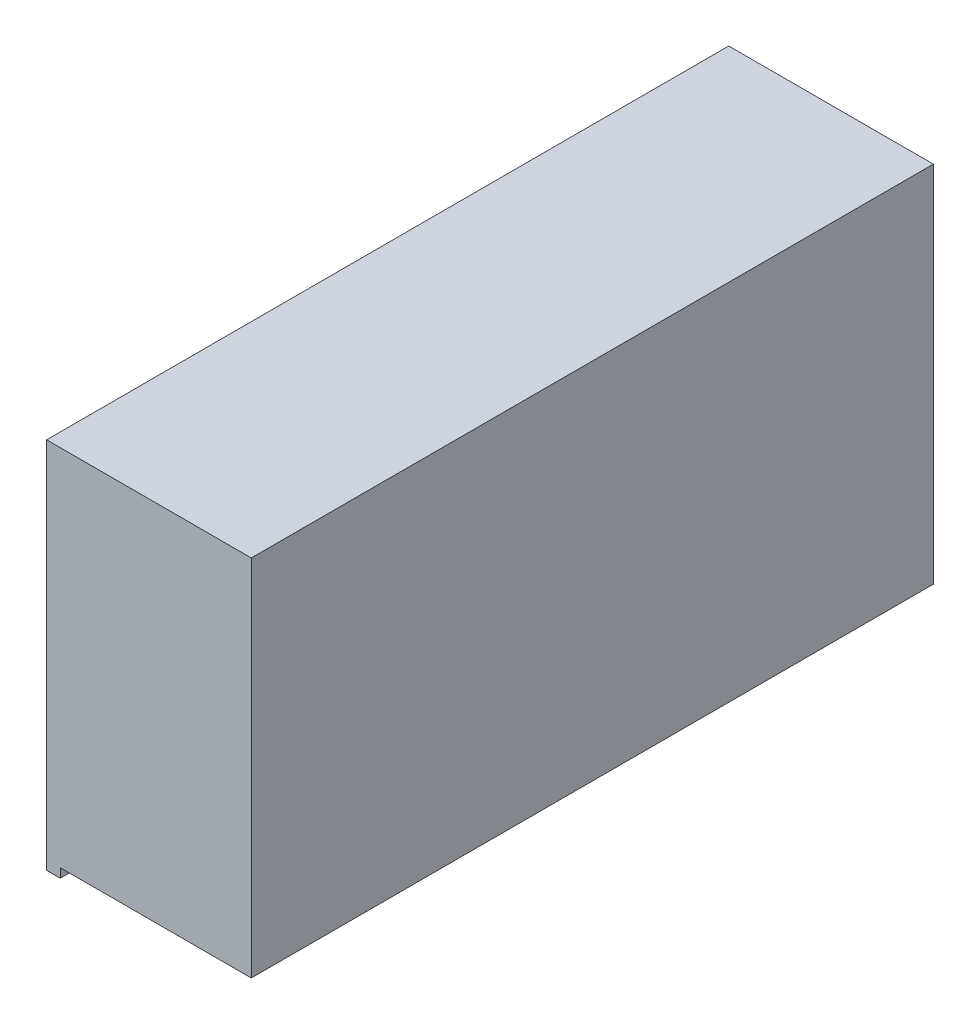
SolidWorks part; units mm, degrees
ref_plane "前视基准面" through (0, 0, 0) normal (0, 0, 1) x (1, 0, 0)
ref_plane "上视基准面" through (0, 0, 0) normal (0, 1, 0) x (1, 0, 0)
ref_plane "右视基准面" through (0, 0, 0) normal (1, 0, 0) x (0, 0, -1)
sketch "草图1" plane through (0, 0, 0) normal (0, 0, 1) x (1, 0, 0)
  line L0 (0, 0) -> (0, 82)
  line L1 (0, 82) -> (45, 82)
  line L2 (45, 82) -> (45, 2)
  line L3 (45, 2) -> (3, 2)
  line L4 (3, 2) -> (3, 0)
  line L5 (3, 0) -> (0, 0)
  dimension "D1" = 3
  dimension "D2" = 42
  dimension "D3" = 2
  dimension "D4" = 80
extrude "凸台-拉伸1" add sketch "草图1" along normal mid plane 150
